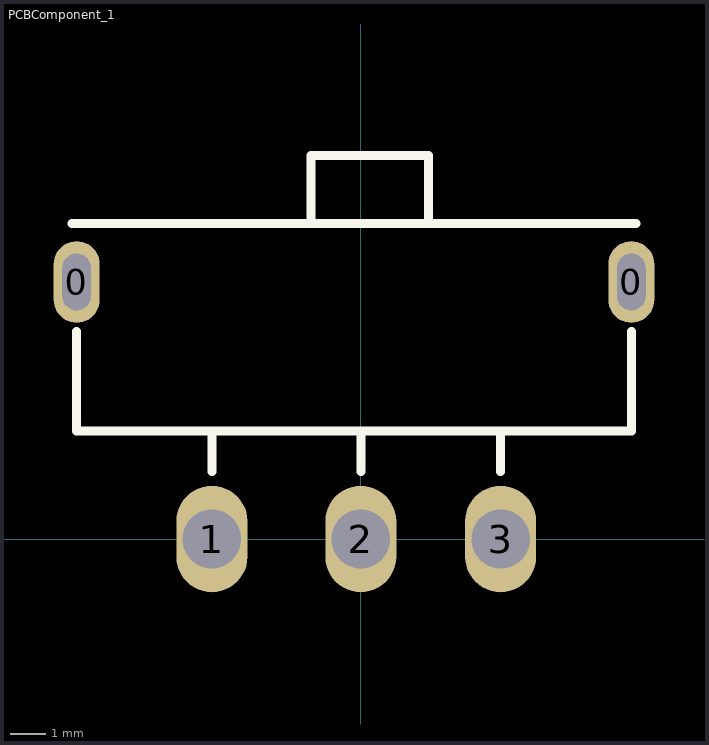
[diagram p0: the footprint, top view; thin cyan lines are the x and y axes]
# Altium footprint library MISC82341-19.PcbLib: 1 footprints
Each footprint in its own frame and in the unit in brackets; x right, y up, seen from the top. Pads: shape width x height; smd on the part's side, far side on the other; paste and mask are expansions set on the pad; w line width, h text height; cw(c..) or ccw(c..) is an arc to the next point about the centre after c.

## PCBComponent_1 [mm]
pads (5):
  oval 1.3x2.3 hole 0.8 slot 1.6 at 90 deg: 0(-8.001,7.239) 0(7.62,7.239)
  oval 2x3 hole 1.65: 1(-4.191,0) 2(0,0) 3(3.937,0)
Top Overlay:
  lines w0.254: -8.128,8.89 7.747,8.89 ; -8.001,5.842 -8.001,3.048 7.62,3.048 7.62,5.461 7.62,5.842 ; -4.191,1.905 -4.191,3.048 ; -1.397,9.017 -1.397,10.795 1.905,10.795 1.905,9.017 ; 0,1.905 0,3.048 ; 3.937,1.905 3.937,3.048